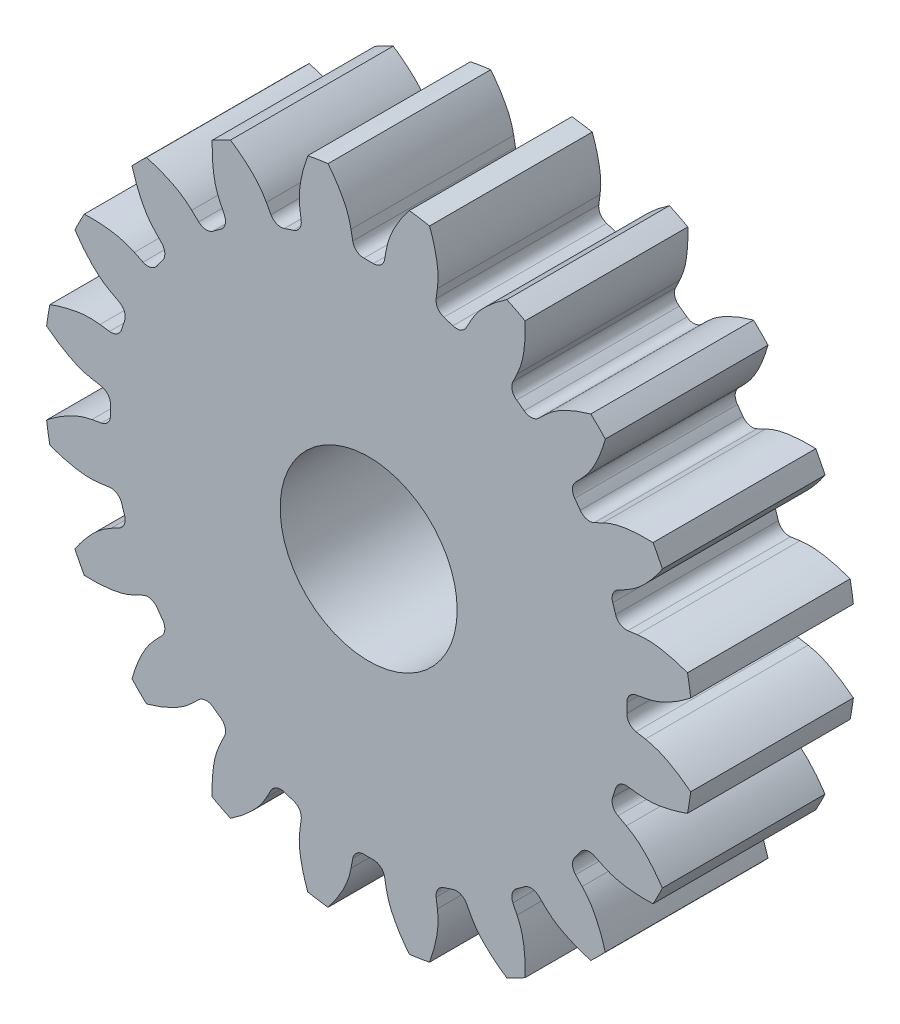
from build123d import *

# Parameters (mm, degrees)
MODEL_R             = 4.5
BOSS_EXTRUDE1_DEPTH = 8.27


with BuildPart() as part:
    # Model → Boss-Extrude1 (new body)
    with BuildSketch(Plane.XY):
        with BuildLine():
            Line((-163.459737479, -18.462565106), (-162.979676853, -18.398057732))
            add(Edge.make_bspline(
                [(-162.979676853, -18.398057732), (-162.77733293, -18.370868092), (-162.358231543, -18.345884581), (-161.722239156, -18.427547579), (-161.073484467, -18.575840313), (-160.643070553, -18.716227587), (-160.427830773, -18.797927164)],
                knots=[0, 0, 0, 0, 0.613977832, 1.254720871, 1.921311366, 2.613663133, 2.613663133, 2.613663133, 2.613663133], degree=3, weights=[1, 1, 1, 1, 1, 1, 1]))
            ThreePointArc((-160.427830773, -18.797927164), (-160.380982671, -19.054258547), (-160.338188414, -19.311297792))
            ThreePointArc((-160.338188414, -19.311297792), (-160.299458676, -19.568980794), (-160.264803115, -19.827243285))
            add(Edge.make_bspline(
                [(-162.568186509, -20.996105521), (-162.367343941, -20.959436693), (-161.961034507, -20.853687973), (-161.381405057, -20.579489391), (-160.810227657, -20.237978396), (-160.444261753, -19.97145695), (-160.264803115, -19.827243285)],
                knots=[0, 0, 0, 0, 0.613977832, 1.254720871, 1.921311366, 2.613663133, 2.613663133, 2.613663133, 2.613663133], degree=3, weights=[1, 1, 1, 1, 1, 1, 1]))
            Line((-162.568186509, -20.996105521), (-163.044685169, -21.083102254))
            ThreePointArc((-163.044685169, -21.083102254), (-163.383357166, -21.282755507), (-163.512209249, -21.654181521))
            ThreePointArc((-163.512209249, -21.654181521), (-163.510586849, -21.773319084), (-163.510046034, -21.892466465))
            ThreePointArc((-163.510046034, -21.892466465), (-163.510586849, -22.011613847), (-163.512209249, -22.130751409))
            ThreePointArc((-163.512209249, -22.130751409), (-163.383357166, -22.502177423), (-163.044685169, -22.701830677))
            Line((-163.044685169, -22.701830677), (-162.568186509, -22.78882741))
            add(Edge.make_bspline(
                [(-162.568186509, -22.78882741), (-162.367343941, -22.825496237), (-161.961034507, -22.931244957), (-161.381405057, -23.20544354), (-160.810227657, -23.546954534), (-160.444261753, -23.81347598), (-160.264803115, -23.957689645)],
                knots=[0, 0, 0, 0, 0.613977832, 1.254720871, 1.921311366, 2.613663133, 2.613663133, 2.613663133, 2.613663133], degree=3, weights=[1, 1, 1, 1, 1, 1, 1]))
            ThreePointArc((-160.264803115, -23.957689645), (-160.299458676, -24.215952136), (-160.338188414, -24.473635138))
            ThreePointArc((-160.338188414, -24.473635138), (-160.380982671, -24.730674384), (-160.427830773, -24.987005766))
            add(Edge.make_bspline(
                [(-162.979676853, -25.386875199), (-162.77733293, -25.414064838), (-162.358231543, -25.439048349), (-161.722239156, -25.357385351), (-161.073484467, -25.209092617), (-160.643070553, -25.068705343), (-160.427830773, -24.987005766)],
                knots=[0, 0, 0, 0, 0.613977832, 1.254720871, 1.921311366, 2.613663133, 2.613663133, 2.613663133, 2.613663133], degree=3, weights=[1, 1, 1, 1, 1, 1, 1]))
            Line((-162.979676853, -25.386875199), (-163.459737479, -25.322367825))
            ThreePointArc((-163.459737479, -25.322367825), (-163.843529937, -25.40759395), (-164.0808525, -25.721023597))
            ThreePointArc((-164.0808525, -25.721023597), (-164.116125037, -25.834831502), (-164.152429258, -25.948314516))
            ThreePointArc((-164.152429258, -25.948314516), (-164.189762169, -26.061463289), (-164.228120695, -26.174268495))
            ThreePointArc((-164.228120695, -26.174268495), (-164.220352032, -26.567333109), (-163.959952071, -26.861870039))
            Line((-163.959952071, -26.861870039), (-163.533658383, -27.091855033))
            add(Edge.make_bspline(
                [(-163.533658383, -27.091855033), (-163.353977041, -27.188792927), (-163.000231958, -27.414922457), (-162.533703615, -27.854816156), (-162.096014327, -28.356115936), (-161.830319726, -28.722682577), (-161.704208893, -28.915293692)],
                knots=[0, 0, 0, 0, 0.613977832, 1.254720871, 1.921311366, 2.613663133, 2.613663133, 2.613663133, 2.613663133], degree=3, weights=[1, 1, 1, 1, 1, 1, 1]))
            ThreePointArc((-161.704208893, -28.915293692), (-161.816975788, -29.15020676), (-161.933438385, -29.383309711))
            ThreePointArc((-161.933438385, -29.383309711), (-162.053567637, -29.614544408), (-162.177333583, -29.843853179))
            add(Edge.make_bspline(
                [(-164.727849876, -29.435587803), (-164.54381143, -29.523974398), (-164.152942655, -29.677244579), (-163.522842696, -29.796110909), (-162.860015347, -29.855552363), (-162.407285336, -29.855041344), (-162.177333583, -29.843853179)],
                knots=[0, 0, 0, 0, 0.613977832, 1.254720871, 1.921311366, 2.613663133, 2.613663133, 2.613663133, 2.613663133], degree=3, weights=[1, 1, 1, 1, 1, 1, 1]))
            Line((-164.727849876, -29.435587803), (-165.164480788, -29.225890753))
            ThreePointArc((-165.164480788, -29.225890753), (-165.555825426, -29.188347223), (-165.878387684, -29.413099826))
            ThreePointArc((-165.878387684, -29.413099826), (-165.947102437, -29.510437762), (-166.016697983, -29.607147901))
            ThreePointArc((-166.016697983, -29.607147901), (-166.087168585, -29.703222275), (-166.158508436, -29.798652965))
            ThreePointArc((-166.158508436, -29.798652965), (-166.272583645, -30.174880276), (-166.115945482, -30.535469556))
            Line((-166.115945482, -30.535469556), (-165.781585364, -30.885930277))
            add(Edge.make_bspline(
                [(-165.781585364, -30.885930277), (-165.64065371, -31.033648282), (-165.374100011, -31.358023486), (-165.066339818, -31.920552442), (-164.804982721, -32.532570292), (-164.665567461, -32.963300032), (-164.605149039, -33.185454479)],
                knots=[0, 0, 0, 0, 0.613977832, 1.254720871, 1.921311366, 2.613663133, 2.613663133, 2.613663133, 2.613663133], degree=3, weights=[1, 1, 1, 1, 1, 1, 1]))
            ThreePointArc((-164.605149039, -33.185454479), (-164.78498886, -33.374023196), (-164.967784144, -33.559728355))
            ThreePointArc((-164.967784144, -33.559728355), (-165.153489303, -33.742523639), (-165.34205802, -33.92236346))
            add(Edge.make_bspline(
                [(-167.641582222, -32.745927135), (-167.493864217, -32.886858789), (-167.169489013, -33.153412488), (-166.606960057, -33.461172681), (-165.994942207, -33.722529778), (-165.564212467, -33.861945038), (-165.34205802, -33.92236346)],
                knots=[0, 0, 0, 0, 0.613977832, 1.254720871, 1.921311366, 2.613663133, 2.613663133, 2.613663133, 2.613663133], degree=3, weights=[1, 1, 1, 1, 1, 1, 1]))
            Line((-167.641582222, -32.745927135), (-167.992042943, -32.411567017))
            ThreePointArc((-167.992042943, -32.411567017), (-168.352632223, -32.254928854), (-168.728859534, -32.369004063))
            ThreePointArc((-168.728859534, -32.369004063), (-168.824290224, -32.440343914), (-168.920364598, -32.510814516))
            ThreePointArc((-168.920364598, -32.510814516), (-169.017074737, -32.580410062), (-169.114412673, -32.649124815))
            ThreePointArc((-169.114412673, -32.649124815), (-169.339165276, -32.971687073), (-169.301621746, -33.363031711))
            Line((-169.301621746, -33.363031711), (-169.091924696, -33.799662623))
            add(Edge.make_bspline(
                [(-169.091924696, -33.799662623), (-169.003538101, -33.983701069), (-168.85026792, -34.374569844), (-168.73140159, -35.004669803), (-168.671960136, -35.667497152), (-168.672471155, -36.120227163), (-168.68365932, -36.350178916)],
                knots=[0, 0, 0, 0, 0.613977832, 1.254720871, 1.921311366, 2.613663133, 2.613663133, 2.613663133, 2.613663133], degree=3, weights=[1, 1, 1, 1, 1, 1, 1]))
            ThreePointArc((-168.68365932, -36.350178916), (-168.912968091, -36.473944862), (-169.144202788, -36.594074114))
            ThreePointArc((-169.144202788, -36.594074114), (-169.377305739, -36.710536711), (-169.612218807, -36.823303606))
            add(Edge.make_bspline(
                [(-171.435657466, -34.993854116), (-171.338719572, -35.173535458), (-171.112590042, -35.527280541), (-170.672696343, -35.993808884), (-170.171396563, -36.431498172), (-169.804829922, -36.697192773), (-169.612218807, -36.823303606)],
                knots=[0, 0, 0, 0, 0.613977832, 1.254720871, 1.921311366, 2.613663133, 2.613663133, 2.613663133, 2.613663133], degree=3, weights=[1, 1, 1, 1, 1, 1, 1]))
            Line((-171.435657466, -34.993854116), (-171.66564246, -34.567560428))
            ThreePointArc((-171.66564246, -34.567560428), (-171.96017939, -34.307160467), (-172.353244004, -34.299391805))
            ThreePointArc((-172.353244004, -34.299391805), (-172.46604921, -34.33775033), (-172.579197983, -34.375083241))
            ThreePointArc((-172.579197983, -34.375083241), (-172.692680997, -34.411387462), (-172.806488902, -34.446659999))
            ThreePointArc((-172.806488902, -34.446659999), (-173.119918549, -34.683982562), (-173.205144674, -35.06777502))
            Line((-173.205144674, -35.06777502), (-173.1406373, -35.547835646))
            add(Edge.make_bspline(
                [(-173.1406373, -35.547835646), (-173.113447661, -35.75017957), (-173.08846415, -36.169280956), (-173.170127148, -36.805273343), (-173.318419882, -37.454028032), (-173.458807156, -37.884441946), (-173.540506733, -38.099681726)],
                knots=[0, 0, 0, 0, 0.613977832, 1.254720871, 1.921311366, 2.613663133, 2.613663133, 2.613663133, 2.613663133], degree=3, weights=[1, 1, 1, 1, 1, 1, 1]))
            ThreePointArc((-173.540506733, -38.099681726), (-173.796838115, -38.146529828), (-174.053877361, -38.189324085))
            ThreePointArc((-174.053877361, -38.189324085), (-174.311560363, -38.228053823), (-174.569822854, -38.262709384))
            add(Edge.make_bspline(
                [(-175.738685089, -35.959325991), (-175.702016262, -36.160168559), (-175.596267542, -36.566477992), (-175.322068959, -37.146107442), (-174.980557965, -37.717284842), (-174.714036519, -38.083250746), (-174.569822854, -38.262709384)],
                knots=[0, 0, 0, 0, 0.613977832, 1.254720871, 1.921311366, 2.613663133, 2.613663133, 2.613663133, 2.613663133], degree=3, weights=[1, 1, 1, 1, 1, 1, 1]))
            Line((-175.738685089, -35.959325991), (-175.825681822, -35.48282733))
            ThreePointArc((-175.825681822, -35.48282733), (-176.025335076, -35.144155333), (-176.39676109, -35.01530325))
            ThreePointArc((-176.39676109, -35.01530325), (-176.515898652, -35.01692565), (-176.635046034, -35.017466465))
            ThreePointArc((-176.635046034, -35.017466465), (-176.754193415, -35.01692565), (-176.873330978, -35.01530325))
            ThreePointArc((-176.873330978, -35.01530325), (-177.244756992, -35.144155333), (-177.444410245, -35.48282733))
            Line((-177.444410245, -35.48282733), (-177.531406979, -35.959325991))
            add(Edge.make_bspline(
                [(-177.531406979, -35.959325991), (-177.568075806, -36.160168559), (-177.673824526, -36.566477992), (-177.948023108, -37.146107442), (-178.289534103, -37.717284842), (-178.556055549, -38.083250746), (-178.700269214, -38.262709384)],
                knots=[0, 0, 0, 0, 0.613977832, 1.254720871, 1.921311366, 2.613663133, 2.613663133, 2.613663133, 2.613663133], degree=3, weights=[1, 1, 1, 1, 1, 1, 1]))
            ThreePointArc((-178.700269214, -38.262709384), (-178.958531705, -38.228053823), (-179.216214707, -38.189324085))
            ThreePointArc((-179.216214707, -38.189324085), (-179.473253953, -38.146529828), (-179.729585335, -38.099681726))
            add(Edge.make_bspline(
                [(-180.129454767, -35.547835646), (-180.156644407, -35.75017957), (-180.181627918, -36.169280956), (-180.09996492, -36.805273343), (-179.951672186, -37.454028032), (-179.811284912, -37.884441946), (-179.729585335, -38.099681726)],
                knots=[0, 0, 0, 0, 0.613977832, 1.254720871, 1.921311366, 2.613663133, 2.613663133, 2.613663133, 2.613663133], degree=3, weights=[1, 1, 1, 1, 1, 1, 1]))
            Line((-180.129454767, -35.547835646), (-180.064947393, -35.06777502))
            ThreePointArc((-180.064947393, -35.06777502), (-180.150173518, -34.683982562), (-180.463603166, -34.446659999))
            ThreePointArc((-180.463603166, -34.446659999), (-180.577411071, -34.411387462), (-180.690894085, -34.375083241))
            ThreePointArc((-180.690894085, -34.375083241), (-180.804042858, -34.33775033), (-180.916848064, -34.299391805))
            ThreePointArc((-180.916848064, -34.299391805), (-181.309912678, -34.307160467), (-181.604449608, -34.567560428))
            Line((-181.604449608, -34.567560428), (-181.834434602, -34.993854116))
            add(Edge.make_bspline(
                [(-181.834434602, -34.993854116), (-181.931372496, -35.173535458), (-182.157502025, -35.527280541), (-182.597395724, -35.993808884), (-183.098695505, -36.431498172), (-183.465262146, -36.697192773), (-183.657873261, -36.823303606)],
                knots=[0, 0, 0, 0, 0.613977832, 1.254720871, 1.921311366, 2.613663133, 2.613663133, 2.613663133, 2.613663133], degree=3, weights=[1, 1, 1, 1, 1, 1, 1]))
            ThreePointArc((-183.657873261, -36.823303606), (-183.892786329, -36.710536711), (-184.12588928, -36.594074114))
            ThreePointArc((-184.12588928, -36.594074114), (-184.357123976, -36.473944862), (-184.586432748, -36.350178916))
            add(Edge.make_bspline(
                [(-184.178167372, -33.799662623), (-184.266553966, -33.983701069), (-184.419824148, -34.374569844), (-184.538690478, -35.004669803), (-184.598131931, -35.667497152), (-184.597620913, -36.120227163), (-184.586432748, -36.350178916)],
                knots=[0, 0, 0, 0, 0.613977832, 1.254720871, 1.921311366, 2.613663133, 2.613663133, 2.613663133, 2.613663133], degree=3, weights=[1, 1, 1, 1, 1, 1, 1]))
            Line((-184.178167372, -33.799662623), (-183.968470322, -33.363031711))
            ThreePointArc((-183.968470322, -33.363031711), (-183.930926791, -32.971687073), (-184.155679395, -32.649124815))
            ThreePointArc((-184.155679395, -32.649124815), (-184.253017331, -32.580410062), (-184.34972747, -32.510814516))
            ThreePointArc((-184.34972747, -32.510814516), (-184.445801844, -32.440343914), (-184.541232534, -32.369004063))
            ThreePointArc((-184.541232534, -32.369004063), (-184.917459845, -32.254928854), (-185.278049125, -32.411567017))
            Line((-185.278049125, -32.411567017), (-185.628509846, -32.745927135))
            add(Edge.make_bspline(
                [(-185.628509846, -32.745927135), (-185.776227851, -32.886858789), (-186.100603055, -33.153412488), (-186.663132011, -33.461172681), (-187.275149861, -33.722529778), (-187.705879601, -33.861945038), (-187.928034048, -33.92236346)],
                knots=[0, 0, 0, 0, 0.613977832, 1.254720871, 1.921311366, 2.613663133, 2.613663133, 2.613663133, 2.613663133], degree=3, weights=[1, 1, 1, 1, 1, 1, 1]))
            ThreePointArc((-187.928034048, -33.92236346), (-188.116602765, -33.742523639), (-188.302307924, -33.559728355))
            ThreePointArc((-188.302307924, -33.559728355), (-188.485103208, -33.374023196), (-188.664943029, -33.185454479))
            add(Edge.make_bspline(
                [(-187.488506704, -30.885930277), (-187.629438358, -31.033648282), (-187.895992057, -31.358023486), (-188.20375225, -31.920552442), (-188.465109347, -32.532570292), (-188.604524607, -32.963300032), (-188.664943029, -33.185454479)],
                knots=[0, 0, 0, 0, 0.613977832, 1.254720871, 1.921311366, 2.613663133, 2.613663133, 2.613663133, 2.613663133], degree=3, weights=[1, 1, 1, 1, 1, 1, 1]))
            Line((-187.488506704, -30.885930277), (-187.154146586, -30.535469556))
            ThreePointArc((-187.154146586, -30.535469556), (-186.997508423, -30.174880276), (-187.111583631, -29.798652965))
            ThreePointArc((-187.111583631, -29.798652965), (-187.182923483, -29.703222275), (-187.253394085, -29.607147901))
            ThreePointArc((-187.253394085, -29.607147901), (-187.32298963, -29.510437762), (-187.391704383, -29.413099826))
            ThreePointArc((-187.391704383, -29.413099826), (-187.714266641, -29.188347223), (-188.10561128, -29.225890753))
            Line((-188.10561128, -29.225890753), (-188.542242191, -29.435587803))
            add(Edge.make_bspline(
                [(-188.542242191, -29.435587803), (-188.726280638, -29.523974398), (-189.117149413, -29.677244579), (-189.747249372, -29.796110909), (-190.410076721, -29.855552363), (-190.862806732, -29.855041344), (-191.092758485, -29.843853179)],
                knots=[0, 0, 0, 0, 0.613977832, 1.254720871, 1.921311366, 2.613663133, 2.613663133, 2.613663133, 2.613663133], degree=3, weights=[1, 1, 1, 1, 1, 1, 1]))
            ThreePointArc((-191.092758485, -29.843853179), (-191.216524431, -29.614544408), (-191.336653683, -29.383309711))
            ThreePointArc((-191.336653683, -29.383309711), (-191.45311628, -29.15020676), (-191.565883175, -28.915293692))
            add(Edge.make_bspline(
                [(-189.736433684, -27.091855033), (-189.916115027, -27.188792927), (-190.26986011, -27.414922457), (-190.736388453, -27.854816156), (-191.17407774, -28.356115936), (-191.439772342, -28.722682577), (-191.565883175, -28.915293692)],
                knots=[0, 0, 0, 0, 0.613977832, 1.254720871, 1.921311366, 2.613663133, 2.613663133, 2.613663133, 2.613663133], degree=3, weights=[1, 1, 1, 1, 1, 1, 1]))
            Line((-189.736433684, -27.091855033), (-189.310139997, -26.861870039))
            ThreePointArc((-189.310139997, -26.861870039), (-189.049740036, -26.567333109), (-189.041971373, -26.174268495))
            ThreePointArc((-189.041971373, -26.174268495), (-189.080329899, -26.061463289), (-189.11766281, -25.948314516))
            ThreePointArc((-189.11766281, -25.948314516), (-189.15396703, -25.834831502), (-189.189239568, -25.721023597))
            ThreePointArc((-189.189239568, -25.721023597), (-189.426562131, -25.40759395), (-189.810354589, -25.322367825))
            Line((-189.810354589, -25.322367825), (-190.290415214, -25.386875199))
            add(Edge.make_bspline(
                [(-190.290415214, -25.386875199), (-190.492759138, -25.414064838), (-190.911860524, -25.439048349), (-191.547852912, -25.357385351), (-192.196607601, -25.209092617), (-192.627021514, -25.068705343), (-192.842261295, -24.987005766)],
                knots=[0, 0, 0, 0, 0.613977832, 1.254720871, 1.921311366, 2.613663133, 2.613663133, 2.613663133, 2.613663133], degree=3, weights=[1, 1, 1, 1, 1, 1, 1]))
            ThreePointArc((-192.842261295, -24.987005766), (-192.889109397, -24.730674384), (-192.931903654, -24.473635138))
            ThreePointArc((-192.931903654, -24.473635138), (-192.970633392, -24.215952136), (-193.005288953, -23.957689645))
            add(Edge.make_bspline(
                [(-190.701905559, -22.78882741), (-190.902748127, -22.825496237), (-191.309057561, -22.931244957), (-191.888687011, -23.20544354), (-192.459864411, -23.546954534), (-192.825830315, -23.81347598), (-193.005288953, -23.957689645)],
                knots=[0, 0, 0, 0, 0.613977832, 1.254720871, 1.921311366, 2.613663133, 2.613663133, 2.613663133, 2.613663133], degree=3, weights=[1, 1, 1, 1, 1, 1, 1]))
            Line((-190.701905559, -22.78882741), (-190.225406899, -22.701830677))
            ThreePointArc((-190.225406899, -22.701830677), (-189.886734902, -22.502177423), (-189.757882819, -22.130751409))
            ThreePointArc((-189.757882819, -22.130751409), (-189.759505219, -22.011613847), (-189.760046034, -21.892466465))
            ThreePointArc((-189.760046034, -21.892466465), (-189.759505219, -21.773319084), (-189.757882819, -21.654181521))
            ThreePointArc((-189.757882819, -21.654181521), (-189.886734902, -21.282755507), (-190.225406899, -21.083102254))
            Line((-190.225406899, -21.083102254), (-190.701905559, -20.996105521))
            add(Edge.make_bspline(
                [(-190.701905559, -20.996105521), (-190.902748127, -20.959436693), (-191.309057561, -20.853687973), (-191.888687011, -20.579489391), (-192.459864411, -20.237978396), (-192.825830315, -19.97145695), (-193.005288953, -19.827243285)],
                knots=[0, 0, 0, 0, 0.613977832, 1.254720871, 1.921311366, 2.613663133, 2.613663133, 2.613663133, 2.613663133], degree=3, weights=[1, 1, 1, 1, 1, 1, 1]))
            ThreePointArc((-193.005288953, -19.827243285), (-192.970633392, -19.568980794), (-192.931903654, -19.311297792))
            ThreePointArc((-192.931903654, -19.311297792), (-192.889109397, -19.054258547), (-192.842261295, -18.797927164))
            add(Edge.make_bspline(
                [(-190.290415214, -18.398057732), (-190.492759138, -18.370868092), (-190.911860524, -18.345884581), (-191.547852912, -18.427547579), (-192.196607601, -18.575840313), (-192.627021514, -18.716227587), (-192.842261295, -18.797927164)],
                knots=[0, 0, 0, 0, 0.613977832, 1.254720871, 1.921311366, 2.613663133, 2.613663133, 2.613663133, 2.613663133], degree=3, weights=[1, 1, 1, 1, 1, 1, 1]))
            Line((-190.290415214, -18.398057732), (-189.810354589, -18.462565106))
            ThreePointArc((-189.810354589, -18.462565106), (-189.426562131, -18.377338981), (-189.189239568, -18.063909333))
            ThreePointArc((-189.189239568, -18.063909333), (-189.15396703, -17.950101429), (-189.11766281, -17.836618414))
            ThreePointArc((-189.11766281, -17.836618414), (-189.080329899, -17.723469641), (-189.041971373, -17.610664435))
            ThreePointArc((-189.041971373, -17.610664435), (-189.049740036, -17.217599821), (-189.310139997, -16.923062891))
            Line((-189.310139997, -16.923062891), (-189.736433684, -16.693077897))
            add(Edge.make_bspline(
                [(-189.736433684, -16.693077897), (-189.916115027, -16.596140003), (-190.26986011, -16.370010474), (-190.736388453, -15.930116775), (-191.17407774, -15.428816995), (-191.439772342, -15.062250353), (-191.565883175, -14.869639238)],
                knots=[0, 0, 0, 0, 0.613977832, 1.254720871, 1.921311366, 2.613663133, 2.613663133, 2.613663133, 2.613663133], degree=3, weights=[1, 1, 1, 1, 1, 1, 1]))
            ThreePointArc((-191.565883175, -14.869639238), (-191.45311628, -14.63472617), (-191.336653683, -14.401623219))
            ThreePointArc((-191.336653683, -14.401623219), (-191.216524431, -14.170388523), (-191.092758485, -13.941079751))
            add(Edge.make_bspline(
                [(-188.542242191, -14.349345127), (-188.726280638, -14.260958533), (-189.117149413, -14.107688351), (-189.747249372, -13.988822021), (-190.410076721, -13.929380568), (-190.862806732, -13.929891586), (-191.092758485, -13.941079751)],
                knots=[0, 0, 0, 0, 0.613977832, 1.254720871, 1.921311366, 2.613663133, 2.613663133, 2.613663133, 2.613663133], degree=3, weights=[1, 1, 1, 1, 1, 1, 1]))
            Line((-188.542242191, -14.349345127), (-188.10561128, -14.559042177))
            ThreePointArc((-188.10561128, -14.559042177), (-187.714266641, -14.596585708), (-187.391704383, -14.371833104))
            ThreePointArc((-187.391704383, -14.371833104), (-187.32298963, -14.274495168), (-187.253394085, -14.177785029))
            ThreePointArc((-187.253394085, -14.177785029), (-187.182923483, -14.081710655), (-187.111583631, -13.986279965))
            ThreePointArc((-187.111583631, -13.986279965), (-186.997508423, -13.610052654), (-187.154146586, -13.249463374))
            Line((-187.154146586, -13.249463374), (-187.488506704, -12.899002653))
            add(Edge.make_bspline(
                [(-187.488506704, -12.899002653), (-187.629438358, -12.751284648), (-187.895992057, -12.426909444), (-188.20375225, -11.864380488), (-188.465109347, -11.252362638), (-188.604524607, -10.821632898), (-188.664943029, -10.599478451)],
                knots=[0, 0, 0, 0, 0.613977832, 1.254720871, 1.921311366, 2.613663133, 2.613663133, 2.613663133, 2.613663133], degree=3, weights=[1, 1, 1, 1, 1, 1, 1]))
            ThreePointArc((-188.664943029, -10.599478451), (-188.485103208, -10.410909734), (-188.302307924, -10.225204576))
            ThreePointArc((-188.302307924, -10.225204576), (-188.116602765, -10.042409291), (-187.928034048, -9.86256947))
            add(Edge.make_bspline(
                [(-185.628509846, -11.039005796), (-185.776227851, -10.898074141), (-186.100603055, -10.631520442), (-186.663132011, -10.323760249), (-187.275149861, -10.062403152), (-187.705879601, -9.922987892), (-187.928034048, -9.86256947)],
                knots=[0, 0, 0, 0, 0.613977832, 1.254720871, 1.921311366, 2.613663133, 2.613663133, 2.613663133, 2.613663133], degree=3, weights=[1, 1, 1, 1, 1, 1, 1]))
            Line((-185.628509846, -11.039005796), (-185.278049125, -11.373365913))
            ThreePointArc((-185.278049125, -11.373365913), (-184.917459845, -11.530004076), (-184.541232534, -11.415928868))
            ThreePointArc((-184.541232534, -11.415928868), (-184.445801844, -11.344589016), (-184.34972747, -11.274118414))
            ThreePointArc((-184.34972747, -11.274118414), (-184.253017331, -11.204522869), (-184.155679395, -11.135808116))
            ThreePointArc((-184.155679395, -11.135808116), (-183.930926791, -10.813245858), (-183.968470322, -10.421901219))
            Line((-183.968470322, -10.421901219), (-184.178167372, -9.985270308))
            add(Edge.make_bspline(
                [(-184.178167372, -9.985270308), (-184.266553966, -9.801231861), (-184.419824148, -9.410363086), (-184.538690478, -8.780263127), (-184.598131931, -8.117435778), (-184.597620913, -7.664705768), (-184.586432748, -7.434754014)],
                knots=[0, 0, 0, 0, 0.613977832, 1.254720871, 1.921311366, 2.613663133, 2.613663133, 2.613663133, 2.613663133], degree=3, weights=[1, 1, 1, 1, 1, 1, 1]))
            ThreePointArc((-184.586432748, -7.434754014), (-184.357123976, -7.310988068), (-184.12588928, -7.190858816))
            ThreePointArc((-184.12588928, -7.190858816), (-183.892786329, -7.074396219), (-183.657873261, -6.961629324))
            add(Edge.make_bspline(
                [(-181.834434602, -8.791078815), (-181.931372496, -8.611397473), (-182.157502025, -8.257652389), (-182.597395724, -7.791124046), (-183.098695505, -7.353434759), (-183.465262146, -7.087740158), (-183.657873261, -6.961629324)],
                knots=[0, 0, 0, 0, 0.613977832, 1.254720871, 1.921311366, 2.613663133, 2.613663133, 2.613663133, 2.613663133], degree=3, weights=[1, 1, 1, 1, 1, 1, 1]))
            Line((-181.834434602, -8.791078815), (-181.604449608, -9.217372502))
            ThreePointArc((-181.604449608, -9.217372502), (-181.309912678, -9.477772463), (-180.916848064, -9.485541126))
            ThreePointArc((-180.916848064, -9.485541126), (-180.804042858, -9.4471826), (-180.690894085, -9.409849689))
            ThreePointArc((-180.690894085, -9.409849689), (-180.577411071, -9.373545469), (-180.463603166, -9.338272931))
            ThreePointArc((-180.463603166, -9.338272931), (-180.150173518, -9.100950368), (-180.064947393, -8.71715791))
            Line((-180.064947393, -8.71715791), (-180.129454767, -8.237097285))
            add(Edge.make_bspline(
                [(-180.129454767, -8.237097285), (-180.156644407, -8.034753361), (-180.181627918, -7.615651975), (-180.09996492, -6.979659587), (-179.951672186, -6.330904898), (-179.811284912, -5.900490985), (-179.729585335, -5.685251204)],
                knots=[0, 0, 0, 0, 0.613977832, 1.254720871, 1.921311366, 2.613663133, 2.613663133, 2.613663133, 2.613663133], degree=3, weights=[1, 1, 1, 1, 1, 1, 1]))
            ThreePointArc((-179.729585335, -5.685251204), (-179.473253953, -5.638403102), (-179.216214707, -5.595608845))
            ThreePointArc((-179.216214707, -5.595608845), (-178.958531705, -5.556879107), (-178.700269214, -5.522223546))
            add(Edge.make_bspline(
                [(-177.531406979, -7.82560694), (-177.568075806, -7.624764372), (-177.673824526, -7.218454938), (-177.948023108, -6.638825488), (-178.289534103, -6.067648088), (-178.556055549, -5.701682184), (-178.700269214, -5.522223546)],
                knots=[0, 0, 0, 0, 0.613977832, 1.254720871, 1.921311366, 2.613663133, 2.613663133, 2.613663133, 2.613663133], degree=3, weights=[1, 1, 1, 1, 1, 1, 1]))
            Line((-177.531406979, -7.82560694), (-177.444410245, -8.3021056))
            ThreePointArc((-177.444410245, -8.3021056), (-177.244756992, -8.640777597), (-176.873330978, -8.76962968))
            ThreePointArc((-176.873330978, -8.76962968), (-176.754193415, -8.76800728), (-176.635046034, -8.767466465))
            ThreePointArc((-176.635046034, -8.767466465), (-176.515898652, -8.76800728), (-176.39676109, -8.76962968))
            ThreePointArc((-176.39676109, -8.76962968), (-176.025335076, -8.640777597), (-175.825681822, -8.3021056))
            Line((-175.825681822, -8.3021056), (-175.738685089, -7.82560694))
            add(Edge.make_bspline(
                [(-175.738685089, -7.82560694), (-175.702016262, -7.624764372), (-175.596267542, -7.218454938), (-175.322068959, -6.638825488), (-174.980557965, -6.067648088), (-174.714036519, -5.701682184), (-174.569822854, -5.522223546)],
                knots=[0, 0, 0, 0, 0.613977832, 1.254720871, 1.921311366, 2.613663133, 2.613663133, 2.613663133, 2.613663133], degree=3, weights=[1, 1, 1, 1, 1, 1, 1]))
            ThreePointArc((-174.569822854, -5.522223546), (-174.311560363, -5.556879107), (-174.053877361, -5.595608845))
            ThreePointArc((-174.053877361, -5.595608845), (-173.796838115, -5.638403102), (-173.540506733, -5.685251204))
            add(Edge.make_bspline(
                [(-173.1406373, -8.237097285), (-173.113447661, -8.034753361), (-173.08846415, -7.615651975), (-173.170127148, -6.979659587), (-173.318419882, -6.330904898), (-173.458807156, -5.900490985), (-173.540506733, -5.685251204)],
                knots=[0, 0, 0, 0, 0.613977832, 1.254720871, 1.921311366, 2.613663133, 2.613663133, 2.613663133, 2.613663133], degree=3, weights=[1, 1, 1, 1, 1, 1, 1]))
            Line((-173.1406373, -8.237097285), (-173.205144674, -8.71715791))
            ThreePointArc((-173.205144674, -8.71715791), (-173.119918549, -9.100950368), (-172.806488902, -9.338272931))
            ThreePointArc((-172.806488902, -9.338272931), (-172.692680997, -9.373545469), (-172.579197983, -9.409849689))
            ThreePointArc((-172.579197983, -9.409849689), (-172.46604921, -9.4471826), (-172.353244004, -9.485541126))
            ThreePointArc((-172.353244004, -9.485541126), (-171.96017939, -9.477772463), (-171.66564246, -9.217372502))
            Line((-171.66564246, -9.217372502), (-171.435657466, -8.791078815))
            add(Edge.make_bspline(
                [(-171.435657466, -8.791078815), (-171.338719572, -8.611397473), (-171.112590042, -8.257652389), (-170.672696343, -7.791124046), (-170.171396563, -7.353434759), (-169.804829922, -7.087740158), (-169.612218807, -6.961629324)],
                knots=[0, 0, 0, 0, 0.613977832, 1.254720871, 1.921311366, 2.613663133, 2.613663133, 2.613663133, 2.613663133], degree=3, weights=[1, 1, 1, 1, 1, 1, 1]))
            ThreePointArc((-169.612218807, -6.961629324), (-169.377305739, -7.074396219), (-169.144202788, -7.190858816))
            ThreePointArc((-169.144202788, -7.190858816), (-168.912968091, -7.310988068), (-168.68365932, -7.434754014))
            add(Edge.make_bspline(
                [(-169.091924696, -9.985270308), (-169.003538101, -9.801231861), (-168.85026792, -9.410363086), (-168.73140159, -8.780263127), (-168.671960136, -8.117435778), (-168.672471155, -7.664705768), (-168.68365932, -7.434754014)],
                knots=[0, 0, 0, 0, 0.613977832, 1.254720871, 1.921311366, 2.613663133, 2.613663133, 2.613663133, 2.613663133], degree=3, weights=[1, 1, 1, 1, 1, 1, 1]))
            Line((-169.091924696, -9.985270308), (-169.301621746, -10.421901219))
            ThreePointArc((-169.301621746, -10.421901219), (-169.339165276, -10.813245858), (-169.114412673, -11.135808116))
            ThreePointArc((-169.114412673, -11.135808116), (-169.017074737, -11.204522869), (-168.920364598, -11.274118414))
            ThreePointArc((-168.920364598, -11.274118414), (-168.824290224, -11.344589016), (-168.728859534, -11.415928868))
            ThreePointArc((-168.728859534, -11.415928868), (-168.352632223, -11.530004076), (-167.992042943, -11.373365913))
            Line((-167.992042943, -11.373365913), (-167.641582222, -11.039005796))
            add(Edge.make_bspline(
                [(-167.641582222, -11.039005796), (-167.493864217, -10.898074141), (-167.169489013, -10.631520442), (-166.606960057, -10.323760249), (-165.994942207, -10.062403152), (-165.564212467, -9.922987892), (-165.34205802, -9.86256947)],
                knots=[0, 0, 0, 0, 0.613977832, 1.254720871, 1.921311366, 2.613663133, 2.613663133, 2.613663133, 2.613663133], degree=3, weights=[1, 1, 1, 1, 1, 1, 1]))
            ThreePointArc((-165.34205802, -9.86256947), (-165.153489303, -10.042409291), (-164.967784144, -10.225204576))
            ThreePointArc((-164.967784144, -10.225204576), (-164.78498886, -10.410909734), (-164.605149039, -10.599478451))
            add(Edge.make_bspline(
                [(-165.781585364, -12.899002653), (-165.64065371, -12.751284648), (-165.374100011, -12.426909444), (-165.066339818, -11.864380488), (-164.804982721, -11.252362638), (-164.665567461, -10.821632898), (-164.605149039, -10.599478451)],
                knots=[0, 0, 0, 0, 0.613977832, 1.254720871, 1.921311366, 2.613663133, 2.613663133, 2.613663133, 2.613663133], degree=3, weights=[1, 1, 1, 1, 1, 1, 1]))
            Line((-165.781585364, -12.899002653), (-166.115945482, -13.249463374))
            ThreePointArc((-166.115945482, -13.249463374), (-166.272583645, -13.610052654), (-166.158508436, -13.986279965))
            ThreePointArc((-166.158508436, -13.986279965), (-166.087168585, -14.081710655), (-166.016697983, -14.177785029))
            ThreePointArc((-166.016697983, -14.177785029), (-165.947102437, -14.274495168), (-165.878387684, -14.371833104))
            ThreePointArc((-165.878387684, -14.371833104), (-165.555825426, -14.596585708), (-165.164480788, -14.559042177))
            Line((-165.164480788, -14.559042177), (-164.727849876, -14.349345127))
            add(Edge.make_bspline(
                [(-164.727849876, -14.349345127), (-164.54381143, -14.260958533), (-164.152942655, -14.107688351), (-163.522842696, -13.988822021), (-162.860015347, -13.929380568), (-162.407285336, -13.929891586), (-162.177333583, -13.941079751)],
                knots=[0, 0, 0, 0, 0.613977832, 1.254720871, 1.921311366, 2.613663133, 2.613663133, 2.613663133, 2.613663133], degree=3, weights=[1, 1, 1, 1, 1, 1, 1]))
            ThreePointArc((-162.177333583, -13.941079751), (-162.053567637, -14.170388523), (-161.933438385, -14.401623219))
            ThreePointArc((-161.933438385, -14.401623219), (-161.816975788, -14.63472617), (-161.704208893, -14.869639238))
            add(Edge.make_bspline(
                [(-163.533658383, -16.693077897), (-163.353977041, -16.596140003), (-163.000231958, -16.370010474), (-162.533703615, -15.930116775), (-162.096014327, -15.428816995), (-161.830319726, -15.062250353), (-161.704208893, -14.869639238)],
                knots=[0, 0, 0, 0, 0.613977832, 1.254720871, 1.921311366, 2.613663133, 2.613663133, 2.613663133, 2.613663133], degree=3, weights=[1, 1, 1, 1, 1, 1, 1]))
            Line((-163.533658383, -16.693077897), (-163.959952071, -16.923062891))
            ThreePointArc((-163.959952071, -16.923062891), (-164.220352032, -17.217599821), (-164.228120695, -17.610664435))
            ThreePointArc((-164.228120695, -17.610664435), (-164.189762169, -17.723469641), (-164.152429258, -17.836618414))
            ThreePointArc((-164.152429258, -17.836618414), (-164.116125037, -17.950101429), (-164.0808525, -18.063909333))
            ThreePointArc((-164.0808525, -18.063909333), (-163.843529937, -18.377338981), (-163.459737479, -18.462565106))
        make_face()
        with Locations((-176.635046034, -21.892466465)):
            Circle(MODEL_R, mode=Mode.SUBTRACT)
    extrude(amount=BOSS_EXTRUDE1_DEPTH)


solid = part.part
